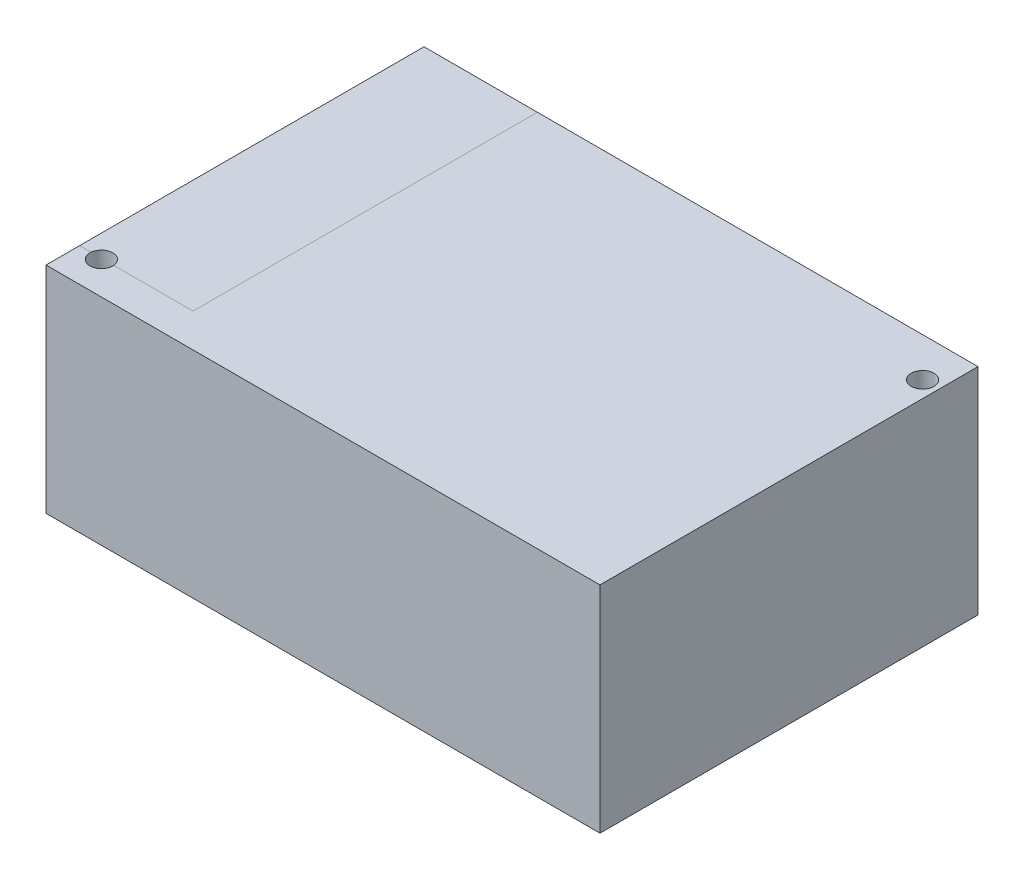
SolidWorks part; units mm, degrees
ref_plane "前视基准面" through (0, 0, 0) normal (0, 0, 1) x (1, 0, 0)
ref_plane "上视基准面" through (0, 0, 0) normal (0, 1, 0) x (1, 0, 0)
ref_plane "右视基准面" through (0, 0, 0) normal (1, 0, 0) x (0, 0, -1)
sketch "草图1" plane through (0, 0, 0) normal (0, 1, 0) x (1, 0, 0)
  line L1 (-42.5, 29) -> (42.5, 29)
  line L2 (-42.5, 29) -> (-42.5, -29)
  line L3 (-42.5, -29) -> (42.5, -29)
  line L4 (42.5, 29) -> (42.5, -29)
  line L5 (-42.5, 29) -> (42.5, -29) construction
  line L6 (-42.5, -29) -> (42.5, 29) construction
  point P0 (0, 0)
  dimension "D1" = 85
  dimension "D2" = 58
extrude "凸台-拉伸1" add sketch "草图1" along normal blind 33
sketch "草图2" plane through (0, 33, 0) normal (0, 1, 0) x (1, 0, 0)
  line L1 (-73.7157, 83.2259) -> (-25.0977, 83.2259)
  line L2 (-73.7157, 83.2259) -> (-73.7157, -23.8451)
  line L3 (-73.7157, -23.8451) -> (-25.0977, -23.8451)
  line L4 (-25.0977, 83.2259) -> (-25.0977, -23.8451)
  line L5 (-73.7157, 83.2259) -> (-25.0977, -23.8451) construction
  line L6 (-73.7157, -23.8451) -> (-25.0977, 83.2259) construction
  point P0 (-49.4067, 29.6904)
split line "分割线1"
hole_wizard "Ø3.5 (3.5) 直径孔1" positions "草图4" profile "草图3" hole size "Ø3.5" standard "GB" end condition through all
sketch "草图4" plane through (0, 0, 0) normal (0, -1, 0) x (-1, 0, 0)
  line L0 (42.5, 29) -> (42.5, -29) construction
  line L1 (-42.5, 29) -> (42.5, 29) construction
  point P0 (39, -24)
  point P2 (-40, 23)
  dimension "D1" = 3.5
  dimension "D2" = 53
  dimension "D3" = 6
  dimension "D4" = 82.5
sketch "草图3" plane through (-39, 0, 24) normal (1, 0, 0) x (0, 0, -1)
  line L0 (0, 0) -> (0, 33)
  line L1 (0, 33) -> (1.75, 33)
  line L2 (1.75, 33) -> (1.75, 0)
  line L5 (1.75, 0) -> (0, 0)
  line L11 (0, -6.35) -> (0, 107.95) construction
  dimension "通孔孔直径" = 3.5
  dimension "通孔孔深度" = 33
